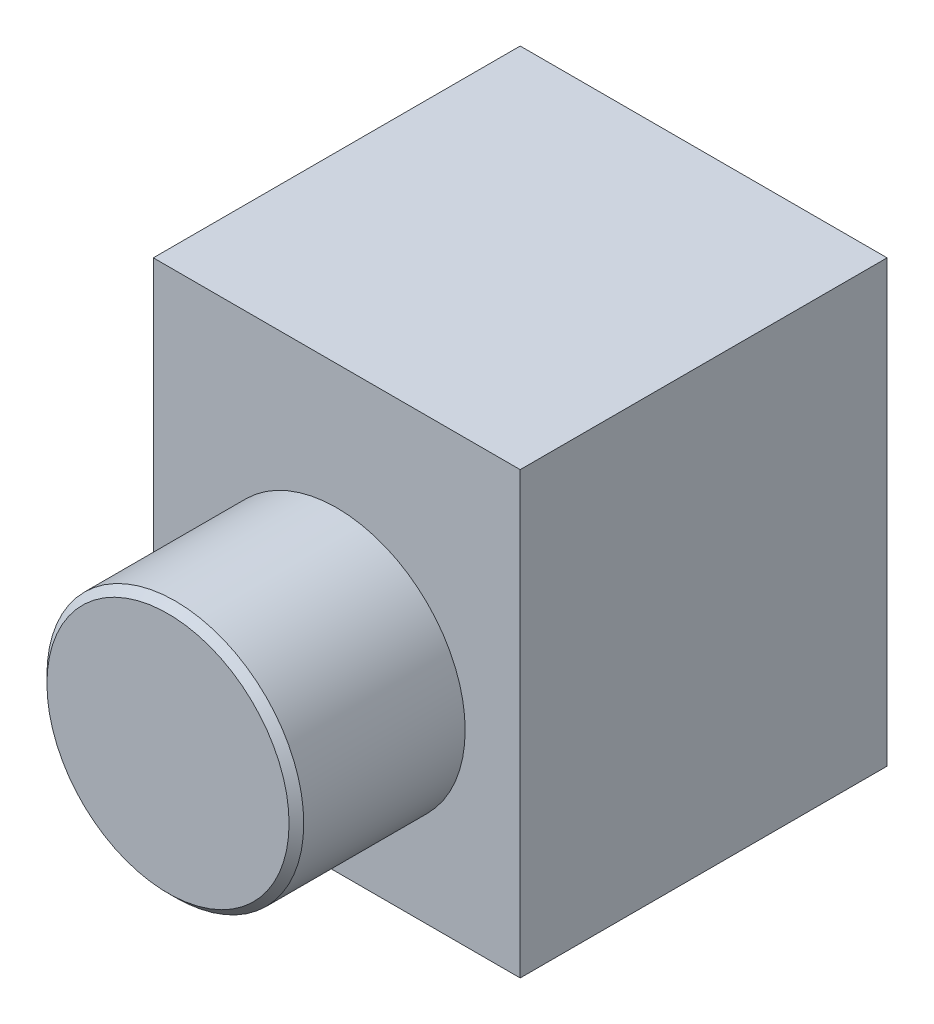
from build123d import *

# Parameters (mm, degrees)
SKETCH_1_W      = 50
SKETCH_1_H      = 60
EXTRUDE_1_DEPTH = 50
SKETCH_2_R      = 17.5
EXTRUDE_2_DEPTH = 23
M30X2_0_1_D     = 28
M30X2_0_1_DEPTH = 20
M30X2_0_1_TIP   = 8.412048666
CHAMFER_1_SIZE  = 1


with BuildPart() as part:
    # 草图1 → 凸台-拉伸1 (new body)
    with BuildSketch(Plane.XY):
        Rectangle(SKETCH_1_W, SKETCH_1_H)
    extrude(amount=EXTRUDE_1_DEPTH)

    # 草图2 → 凸台-拉伸2 (add)
    with BuildSketch(Plane.XY.offset(50)):
        with Locations((0, -4.5)):
            Circle(SKETCH_2_R)
    extrude(amount=EXTRUDE_2_DEPTH)

    # M30x2.0 螺纹孔1
    with Locations(Plane(origin=(0, -30, 0), x_dir=(-1, 0, 0), z_dir=(0, -1, 0))):
        with Locations((0, -25)):
            Hole(M30X2_0_1_D / 2, depth=M30X2_0_1_DEPTH)
            with Locations((0, 0, -(M30X2_0_1_DEPTH + M30X2_0_1_TIP / 2))):  # 118° drill point
                Cone(0, M30X2_0_1_D / 2, M30X2_0_1_TIP, mode=Mode.SUBTRACT)

    # 倒角1
    chamfer_1_edges = [part.edges().sort_by_distance(p)[0] for p in [
        (-17.5, -4.5, 73),
    ]]
    chamfer(chamfer_1_edges, length=CHAMFER_1_SIZE)


solid = part.part
